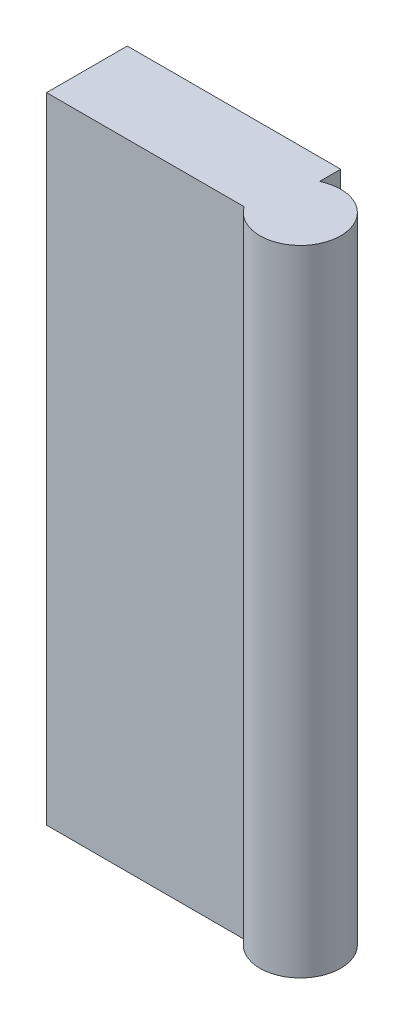
SolidWorks part; units mm, degrees
ref_plane "前视基准面" through (0, 0, 0) normal (0, 0, 1) x (1, 0, 0)
ref_plane "上视基准面" through (0, 0, 0) normal (0, 1, 0) x (1, 0, 0)
ref_plane "右视基准面" through (0, 0, 0) normal (1, 0, 0) x (0, 0, -1)
sketch "草图1" plane through (0, 0, 0) normal (0, 0, 1) x (1, 0, 0)
  line L1 (0, 0) -> (18.5, 0)
  line L2 (0, 0) -> (0, 55)
  line L3 (0, 55) -> (18.5, 55)
  line L4 (18.5, 0) -> (18.5, 55)
  dimension "D1" = 55
  dimension "D2" = 18.5
extrude "凸台-拉伸1" add sketch "草图1" along normal blind 7
sketch "草图2" plane through (0, 55, 0) normal (0, 1, 0) x (1, 0, 0)
  line L0 (18.5, -7) -> (18.5, 0) construction
  line L1 (18.5, 0) -> (0, 0) construction
  circle A0 centre (20, -5) radius 3.5
  dimension "D1" = 7
  dimension "D2" = 1.5
  dimension "D3" = 5
extrude "凸台-拉伸2" add sketch "草图2" against normal up to surface (55 mm away) up to face at (9.25, 0, 3.5)
